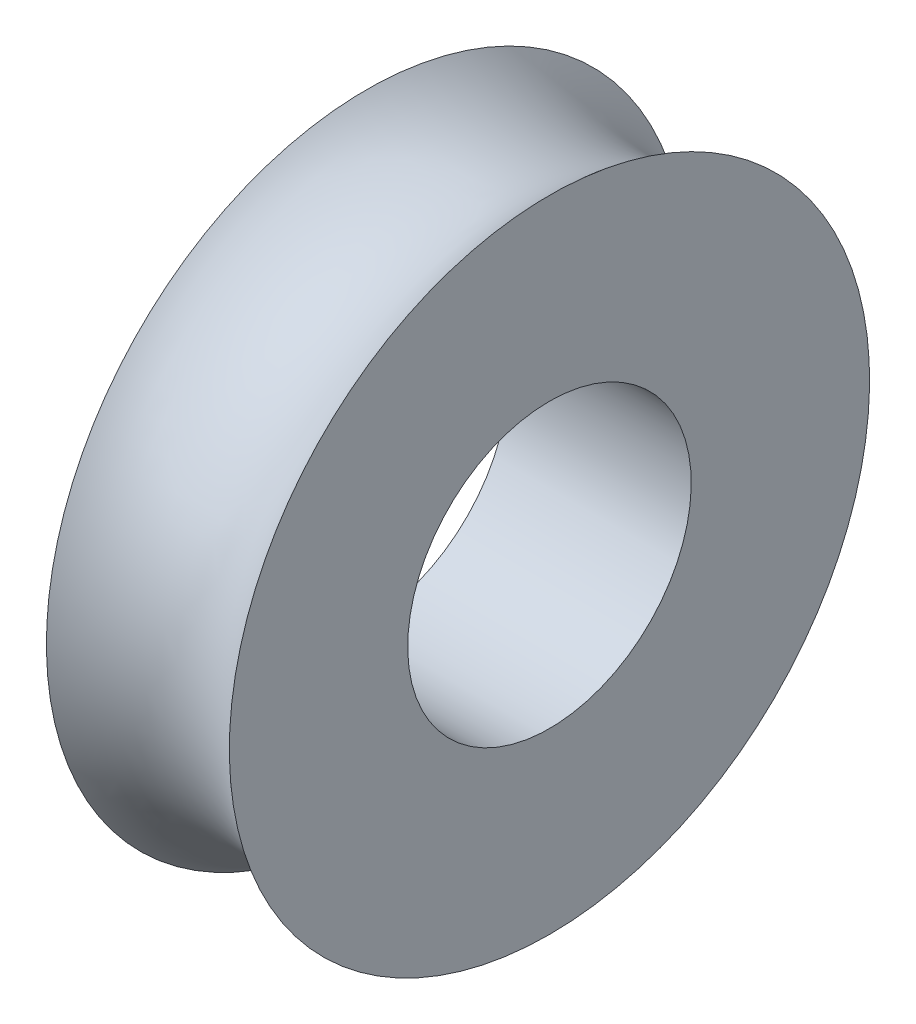
SolidWorks part; units mm, degrees
ref_plane "前视基准面" through (0, 0, 0) normal (0, 0, 1) x (1, 0, 0)
ref_plane "上视基准面" through (0, 0, 0) normal (0, 1, 0) x (1, 0, 0)
ref_plane "右视基准面" through (0, 0, 0) normal (1, 0, 0) x (0, 0, -1)
sketch "草图1" plane through (0, 0, 0) normal (0, 0, 1) x (1, 0, 0)
  line L0 (-20, 0) -> (20, 0) construction
  line L1 (-20, 70) -> (-20, 0)
  line L2 (20, 70) -> (20, 0)
  line L3 (20, 0) -> (-20, 0)
  arc A1 (-20, 70) -> (20, 70) centre (0, 92.3607) ccw
  point P1 (0, 0)
  point P6 (0, 0)
  dimension "D1" = 40
  dimension "D3" = 30
  dimension "D2" = 70
revolve "旋转1" add sketch "草图1" angle 360 about L0
sketch "草图2" plane through (20, 0, 0) normal (1, 0, 0) x (0, 0, -1)
  circle A0 centre (0, 0) radius 31
  dimension "D1" = 62
extrude "切除-拉伸1" cut sketch "草图2" against normal through all
